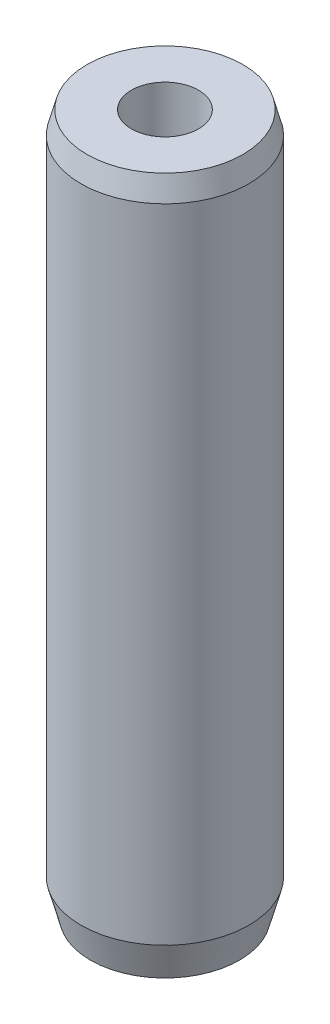
from build123d import *

# Parameters (mm, degrees)
SKETCH1_R             = 6
BOSS_EXTRUDE1_DEPTH   = 25
M6_TAPPED_HOLE1_D     = 4.8
M6_TAPPED_HOLE1_DEPTH = 20
M6_TAPPED_HOLE1_TIP   = 1.385640646
CHAMFER1_SIZE         = 1.6
CHAMFER1_SIZE2        = 0.428718708
CHAMFER2_SIZE         = 2.5
CHAMFER2_SIZE2        = 0.669872981


with BuildPart() as part:
    # Sketch1 → Boss-Extrude1 (new, symmetric)
    with BuildSketch(Plane(origin=(0, 0, 0), x_dir=(1, 0, 0), z_dir=(0, 1, 0))):
        with Locations(Location((0, 0, 0), (0, 0, 270))):
            Circle(SKETCH1_R)
    extrude(amount=BOSS_EXTRUDE1_DEPTH, both=True)

    # M6 Tapped Hole1
    with Locations(Plane(origin=(0, 25, 0), x_dir=(1, 0, 0), z_dir=(0, 1, 0))):
        with Locations((0, 0)):
            Hole(M6_TAPPED_HOLE1_D / 2, depth=M6_TAPPED_HOLE1_DEPTH)
            with Locations((0, 0, -(M6_TAPPED_HOLE1_DEPTH + M6_TAPPED_HOLE1_TIP / 2))):  # 120° drill point
                Cone(0, M6_TAPPED_HOLE1_D / 2, M6_TAPPED_HOLE1_TIP, mode=Mode.SUBTRACT)

    # Chamfer1
    chamfer1_edges = [part.edges().sort_by_distance(p)[0] for p in [
        (0, 25, -6),
    ]]
    chamfer1_side = [part.faces().sort_by_distance(p)[0] for p in [
        (0, 0, -6),
    ]]
    chamfer(chamfer1_edges, length=CHAMFER1_SIZE, length2=CHAMFER1_SIZE2, reference=chamfer1_side[0])

    # Chamfer2
    chamfer2_edges = [part.edges().sort_by_distance(p)[0] for p in [
        (0, -25, -6),
    ]]
    chamfer2_side = [part.faces().sort_by_distance(p)[0] for p in [
        (0, -0.8, -6),
    ]]
    chamfer(chamfer2_edges, length=CHAMFER2_SIZE, length2=CHAMFER2_SIZE2, reference=chamfer2_side[0])


solid = part.part
